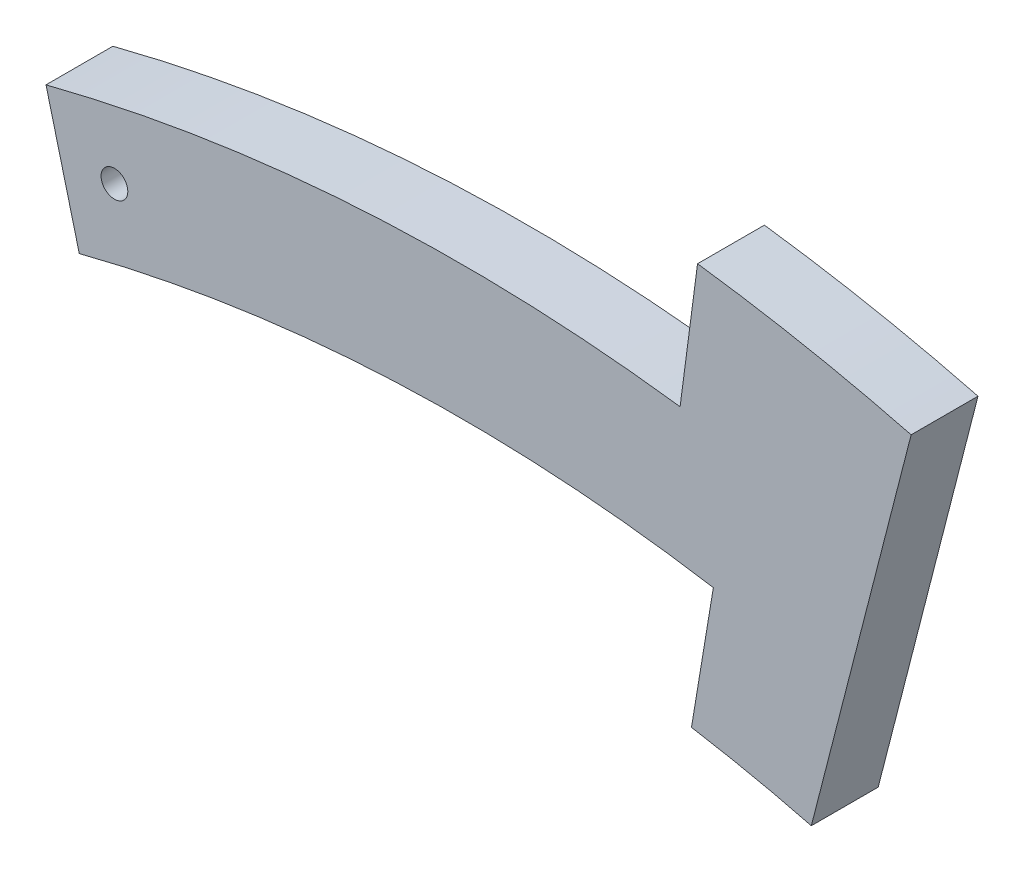
SolidWorks part; units mm, degrees
ref_plane "Front Plane" through (0, 0, 0) normal (0, 0, 1) x (1, 0, 0)
ref_plane "Top Plane" through (0, 0, 0) normal (0, 1, 0) x (1, 0, 0)
ref_plane "Right Plane" through (0, 0, 0) normal (1, 0, 0) x (0, 0, -1)
sketch "Sketch1" plane through (0, 0, 0) normal (0, 0, 1) x (1, 0, 0)
  line L2 (28.6188, 111.3821) -> (31.1074, 121.0675)
  line L3 (18.8023, 113.4525) -> (17.1673, 103.5871)
  line L4 (-28.6188, 111.3821) -> (-31.1074, 121.0675)
  line L5 (31.1074, 121.0675) -> (33.596, 130.7529)
  line L6 (33.596, 130.7529) -> (26.1302, 101.6967)
  line L9 (16.3158, 123.9306) -> (17.621, 133.8451)
  arc A1 (16.3158, 123.9306) -> (-31.1074, 121.0675) centre (0, 0) ccw
  arc A2 (18.8023, 113.4525) -> (-28.6188, 111.3821) centre (0, 0) ccw
  arc A3 (22.0723, 133.1834) -> (33.596, 130.7529) centre (0, 0) cw
  arc A4 (17.1673, 103.5871) -> (26.1302, 101.6967) centre (0, 0) cw
  arc A5 (17.621, 133.8451) -> (22.0723, 133.1834) centre (0, 0) cw
  dimension "D2" = 250
  dimension "D3" = 230
  dimension "D5" = 135
  dimension "D6" = 30
  dimension "D7" = 30
  dimension "D9" = 10
extrude "Boss-Extrude3" add sketch "Sketch1" along normal blind 5 contours A5 L9 A1 L4 A2 L3 A4 L6 L2 L5 A3
sketch "Sketch3" plane through (0, 0, 0) normal (0, 0, -1) x (-1, 0, 0)
  circle A0 centre (25.9889, 117.2202) radius 1
  dimension "D2" = 2
extrude "Cut-Extrude1" cut sketch "Sketch3" against normal blind 10
